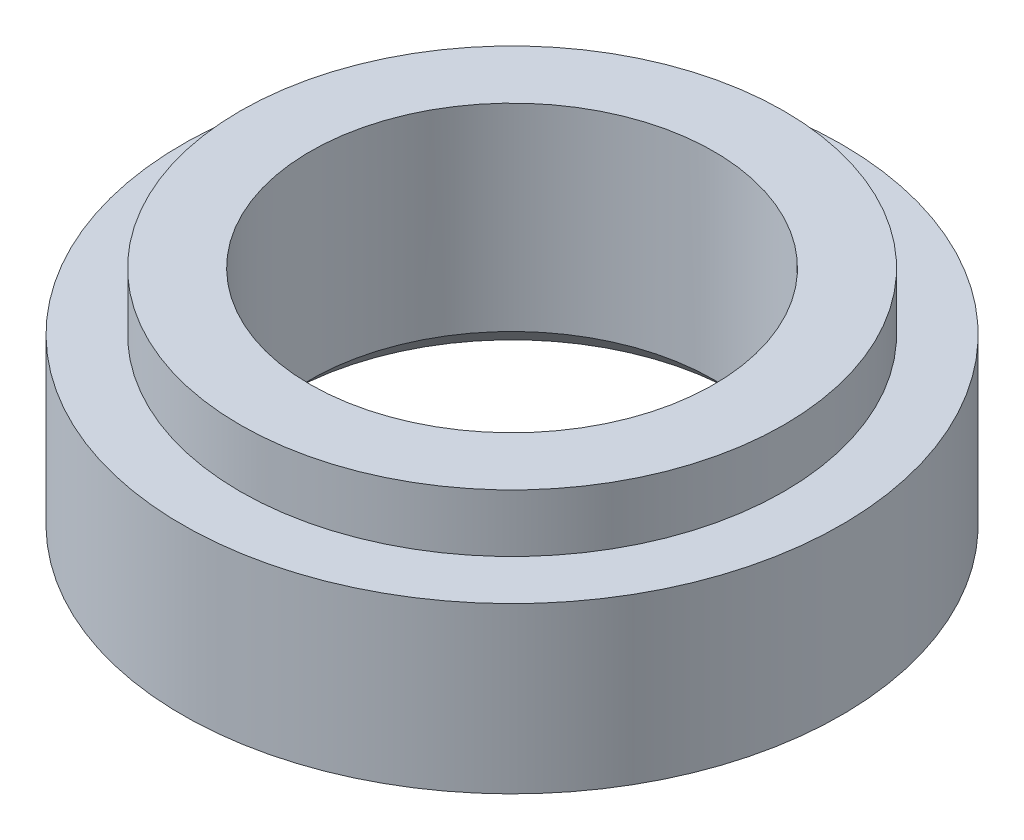
from build123d import *

# Parameters (mm, degrees)
G3_4_TAPPED_HOLE1_D     = 24.5
G3_4_TAPPED_HOLE1_DEPTH = 58.32
G3_4_TAPPED_HOLE1_TIP   = 7.360542583
CHAMFER1_SIZE           = 1.5


with BuildPart() as part:
    # Sketch1 → Revolve1 (revolve)
    with BuildSketch(Plane.XY, mode=Mode.PRIVATE) as revolve1_sk:
        Polygon((0, 0), (20, 0), (20, 10), (16.5, 10), (16.5, 13.5), (0, 13.5), align=None)
    revolve(revolve1_sk.sketch.rotate(Axis((0, 0, 0), (0, 1, 0)), 90), axis=Axis((0, 0, 0), (0, 1, 0)))

    # G3/4 Tapped Hole1
    with Locations(Plane(origin=(0, 13.5, 0), x_dir=(1, 0, 0), z_dir=(0, 1, 0))):
        with Locations((0, 0)):
            Hole(G3_4_TAPPED_HOLE1_D / 2, depth=G3_4_TAPPED_HOLE1_DEPTH)
            with Locations((0, 0, -(G3_4_TAPPED_HOLE1_DEPTH + G3_4_TAPPED_HOLE1_TIP / 2))):  # 118° drill point
                Cone(0, G3_4_TAPPED_HOLE1_D / 2, G3_4_TAPPED_HOLE1_TIP, mode=Mode.SUBTRACT)

    # Chamfer1
    chamfer1_edges = [part.edges().sort_by_distance(p)[0] for p in [
        (12.25, 0, 0),
    ]]
    chamfer(chamfer1_edges, length=CHAMFER1_SIZE)


solid = part.part
